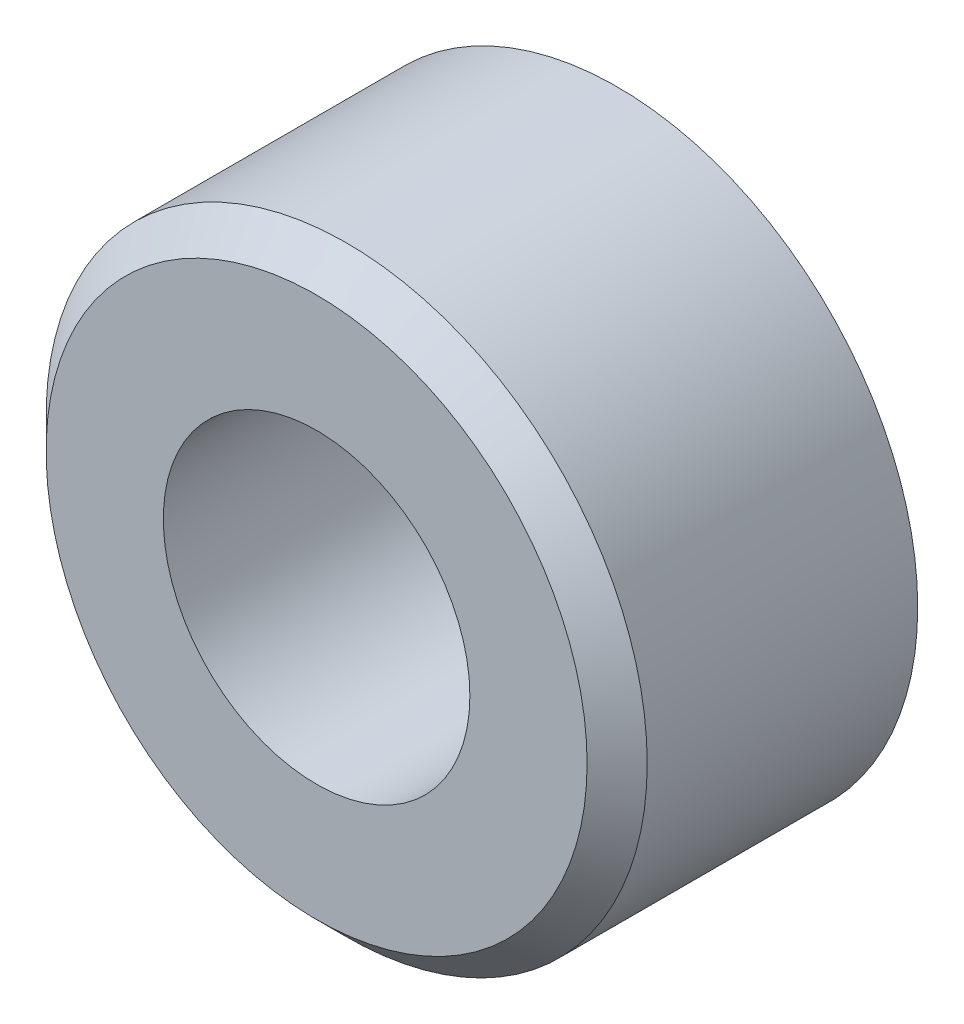
from build123d import *

# Parameters (mm, degrees)
SKETCH_1_R              = 10
EXTRUDE_1_DEPTH         = 10
HOLE_WIZARD_M12_1_D     = 10.2
HOLE_WIZARD_M12_1_DEPTH = 30.25
HOLE_WIZARD_M12_1_TIP   = 3.064389157
CHAMFER_1_SIZE          = 1


with BuildPart() as part:
    # 草图1 → 凸台-拉伸1 (new body)
    with BuildSketch(Plane.XY):
        Circle(SKETCH_1_R)
    extrude(amount=EXTRUDE_1_DEPTH)

    # M12 螺纹孔1
    with Locations(Plane.XY.offset(10)):
        with Locations((0, 0)):
            Hole(HOLE_WIZARD_M12_1_D / 2, depth=HOLE_WIZARD_M12_1_DEPTH)
            with Locations((0, 0, -(HOLE_WIZARD_M12_1_DEPTH + HOLE_WIZARD_M12_1_TIP / 2))):  # 118° drill point
                Cone(0, HOLE_WIZARD_M12_1_D / 2, HOLE_WIZARD_M12_1_TIP, mode=Mode.SUBTRACT)

    # 倒角1
    chamfer_1_edges = [part.edges().sort_by_distance(p)[0] for p in [
        (-10, 0, 10),
    ]]
    chamfer(chamfer_1_edges, length=CHAMFER_1_SIZE)


solid = part.part
